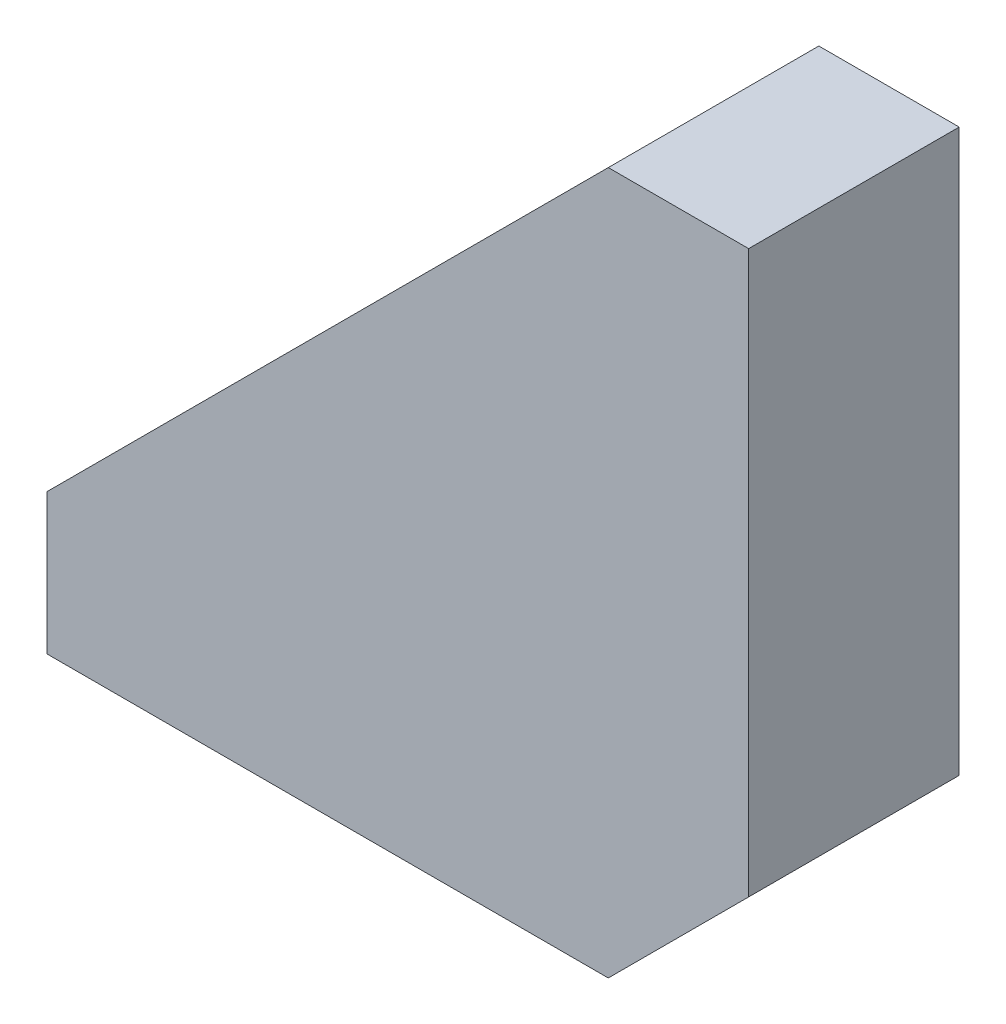
from build123d import *

# Parameters (mm, degrees)
BOSS_EXTRUDE1_DEPTH = 7.5


with BuildPart() as part:
    # Sketch1 → Boss-Extrude1 (new, symmetric)
    with BuildSketch(Plane.XY):
        Polygon((0, 0), (0, 10), (40, 50), (50, 50), (50, 10), (40, 0), align=None)
    extrude(amount=BOSS_EXTRUDE1_DEPTH, both=True)


solid = part.part
